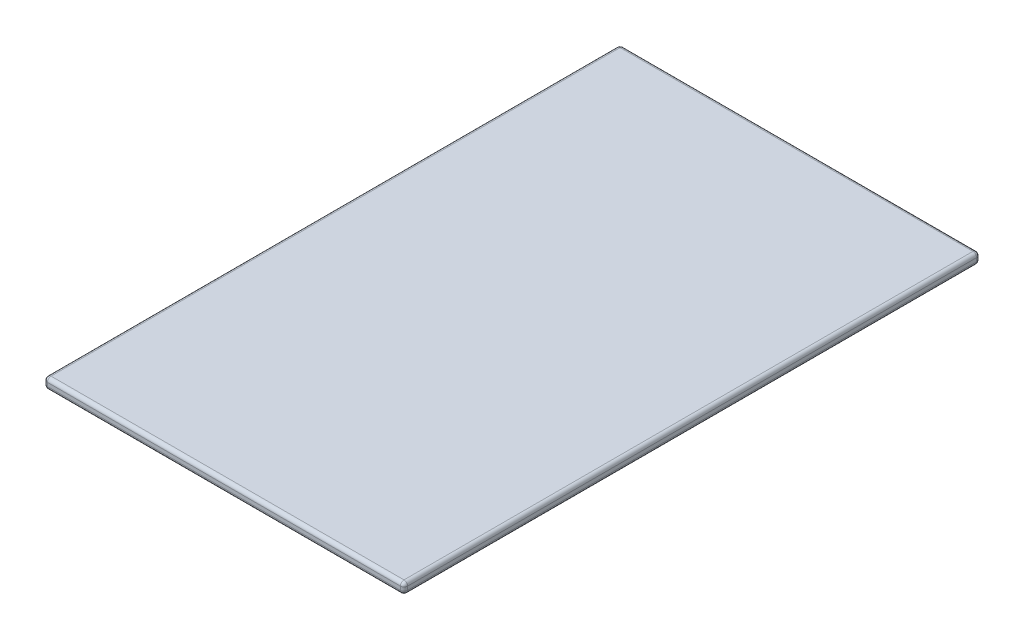
SolidWorks part; units mm, degrees
ref_plane "Front Plane" through (0, 0, 0) normal (0, 0, 1) x (1, 0, 0)
ref_plane "Top Plane" through (0, 0, 0) normal (0, 1, 0) x (1, 0, 0)
ref_plane "Right Plane" through (0, 0, 0) normal (1, 0, 0) x (0, 0, -1)
sketch "Sketch1" plane through (0, 0, 0) normal (0, 1, 0) x (1, 0, 0)
  line L1 (-500, 800) -> (500, 800)
  line L2 (-500, 800) -> (-500, -800)
  line L3 (-500, -800) -> (500, -800)
  line L4 (500, 800) -> (500, -800)
  line L5 (-500, 800) -> (500, -800) construction
  line L6 (-500, -800) -> (500, 800) construction
  point P0 (0, 0)
  dimension "D1" = 1600
  dimension "D2" = 1000
extrude "Boss-Extrude1" add sketch "Sketch1" along normal blind 30
fillet "Fillet3" radius 10 12 edges at (-500, 30, 0) (-500, 0, 0) (0, 30, -800) (-500, 15, -800) (0, 0, -800) (-500, 15, 800) (0, 30, 800) (0, 0, 800) (500, 15, 800) (500, 30, 0) (500, 15, -800) (500, 0, 0)
